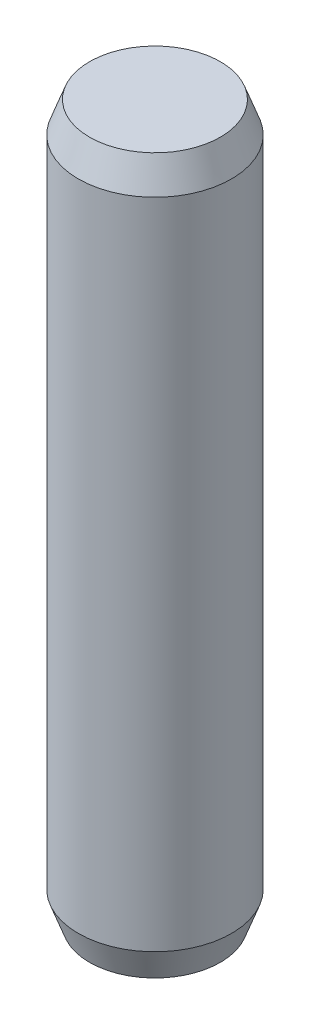
from build123d import *

# Parameters (mm, degrees)
SKETCH1_R           = 3
BOSS_EXTRUDE1_DEPTH = 14
CHAMFER1_SIZE       = 1.2
CHAMFER1_SIZE2      = 0.436764281
CHAMFER2_SIZE       = 1.2
CHAMFER2_SIZE2      = 0.436764281


with BuildPart() as part:
    # Sketch1 → Boss-Extrude1 (new, symmetric)
    with BuildSketch(Plane(origin=(0, 0, 0), x_dir=(1, 0, 0), z_dir=(0, 1, 0))):
        with Locations(Location((0, 0, 0), (0, 0, 270))):
            Circle(SKETCH1_R)
    extrude(amount=BOSS_EXTRUDE1_DEPTH, both=True)

    # Chamfer1
    chamfer1_edges = [part.edges().sort_by_distance(p)[0] for p in [
        (0, 14, -3),
    ]]
    chamfer1_side = [part.faces().sort_by_distance(p)[0] for p in [
        (0, 0, -3),
    ]]
    chamfer(chamfer1_edges, length=CHAMFER1_SIZE, length2=CHAMFER1_SIZE2, reference=chamfer1_side[0])

    # Chamfer2
    chamfer2_edges = [part.edges().sort_by_distance(p)[0] for p in [
        (0, -14, -3),
    ]]
    chamfer2_side = [part.faces().sort_by_distance(p)[0] for p in [
        (0, -0.6, -3),
    ]]
    chamfer(chamfer2_edges, length=CHAMFER2_SIZE, length2=CHAMFER2_SIZE2, reference=chamfer2_side[0])


solid = part.part
